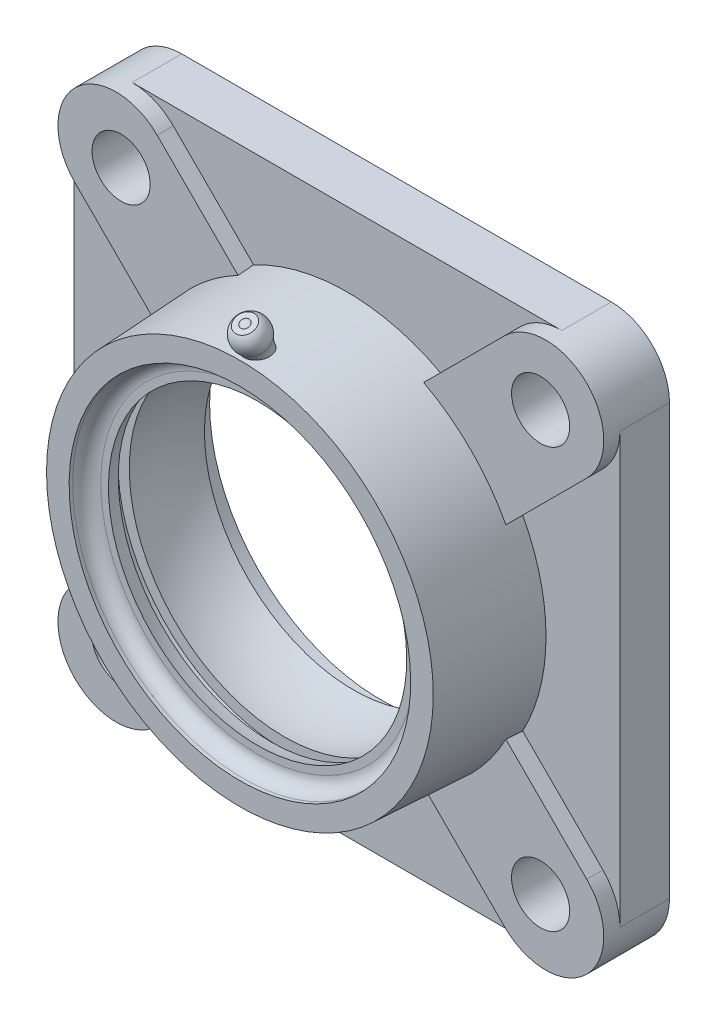
from build123d import *

# Parameters (mm, degrees)
SKETCH_1_R          = 5.75
EXTRUDE_686_DEPTH   = 9.8
SKETCH_2_R          = 5.75
EXTRUDE_1_DEPTH     = 13
CUT_EXTRUDE_3_DEPTH = 3.2
SKETCH_4_R          = 39.37
EXTRUDE_2_DEPTH     = 21.2
EXTRUDE_2_TAPER     = 3


with BuildPart() as part:
    # 草图1 → Extrude 686 (new body)
    with BuildSketch(Plane.XY):
        with BuildLine():
            Line((-42.5, -54), (42.5, -54))
            ThreePointArc((42.5, -54), (50.631727984, -50.631727984), (54, -42.5))
            Line((54, -42.5), (54, 42.5))
            ThreePointArc((54, 42.5), (50.631727984, 50.631727984), (42.5, 54))
            Line((42.5, 54), (-42.5, 54))
            ThreePointArc((-42.5, 54), (-50.631727984, 50.631727984), (-54, 42.5))
            Line((-54, 42.5), (-54, -42.5))
            ThreePointArc((-54, -42.5), (-50.631727984, -50.631727984), (-42.5, -54))
        make_face()
        with Locations((-41.5, -41.5)):
            Circle(SKETCH_1_R, mode=Mode.SUBTRACT)
        with Locations(Location((-41.5, 41.5, 0), (0, 0, 180))):
            Circle(SKETCH_1_R, mode=Mode.SUBTRACT)
        with Locations(Location((41.5, -41.5, 0), (0, 0, 180))):
            Circle(SKETCH_1_R, mode=Mode.SUBTRACT)
        with Locations((41.5, 41.5)):
            Circle(SKETCH_1_R, mode=Mode.SUBTRACT)
    extrude(amount=EXTRUDE_686_DEPTH)

    # 草图2 → 凸台-拉伸1 (add)
    # profile 1 of 4: a face of its own
    with BuildSketch(Plane.XY):
        with BuildLine():
            Line((-50.631727984, -34.368272016), (-18.763455967, -2.5))
            Line((-18.763455967, -2.5), (-2.5, -18.763455967))
            Line((-2.5, -18.763455967), (-34.368272016, -50.631727984))
            ThreePointArc((-34.368272016, -50.631727984), (-50.631727984, -50.631727984), (-50.631727984, -34.368272016))
        make_face()
        with Locations((-41.5, -41.5)):
            Circle(SKETCH_2_R, mode=Mode.SUBTRACT)
    # profile 2 of 4: a face of its own
    with BuildSketch(Plane.XY):
        with BuildLine():
            Line((-18.763455967, 2.5), (-2.5, 18.763455967))
            Line((-2.5, 18.763455967), (-34.368272016, 50.631727984))
            ThreePointArc((-34.368272016, 50.631727984), (-50.631727984, 50.631727984), (-50.631727984, 34.368272016))
            Line((-50.631727984, 34.368272016), (-18.763455967, 2.5))
        make_face()
        with Locations(Location((-41.5, 41.5, 0), (0, 0, 180))):
            Circle(SKETCH_2_R, mode=Mode.SUBTRACT)
    # profile 3 of 4: a face of its own
    with BuildSketch(Plane.XY):
        with BuildLine():
            Line((2.5, -18.763455967), (34.368272016, -50.631727984))
            ThreePointArc((34.368272016, -50.631727984), (50.631727984, -50.631727984), (50.631727984, -34.368272016))
            Line((50.631727984, -34.368272016), (18.763455967, -2.5))
            Line((18.763455967, -2.5), (2.5, -18.763455967))
        make_face()
        with Locations(Location((41.5, -41.5, 0), (0, 0, 180))):
            Circle(SKETCH_2_R, mode=Mode.SUBTRACT)
    # profile 4 of 4: a face of its own
    with BuildSketch(Plane.XY):
        with BuildLine():
            Line((2.5, 18.763455967), (34.368272016, 50.631727984))
            ThreePointArc((34.368272016, 50.631727984), (50.631727984, 50.631727984), (50.631727984, 34.368272016))
            Line((50.631727984, 34.368272016), (18.763455967, 2.5))
            Line((18.763455967, 2.5), (2.5, 18.763455967))
        make_face()
        with Locations((41.5, 41.5)):
            Circle(SKETCH_2_R, mode=Mode.SUBTRACT)
    extrude(amount=EXTRUDE_1_DEPTH)

    # 草图3 → 切除-拉伸3 (cut)
    with BuildSketch(Plane.XY):
        with BuildLine():
            Line((-26.757388349, 48.125), (26.757388349, 48.125))
            ThreePointArc((26.757388349, 48.125), (29.193644663, 46.875615655), (29.600687311, 44.168103448))
            ThreePointArc((29.600687311, 44.168103448), (30.719443759, 34.450973663), (38.913793103, 29.10991889))
            ThreePointArc((38.913793103, 29.10991889), (40.762894088, 28.108189877), (41.5, 26.138593384))
            Line((41.5, 26.138593384), (41.5, 12.625))
            ThreePointArc((41.5, 12.625), (42.378679656, 10.503679656), (44.5, 9.625))
            Line((44.5, 9.625), (45.125, 9.625))
            ThreePointArc((45.125, 9.625), (47.246320344, 8.746320344), (48.125, 6.625))
            Line((48.125, 6.625), (48.125, -26.757388349))
            ThreePointArc((48.125, -26.757388349), (46.875615655, -29.193644663), (44.168103448, -29.600687311))
            ThreePointArc((44.168103448, -29.600687311), (32.368272016, -32.368272016), (29.600687311, -44.168103448))
            ThreePointArc((29.600687311, -44.168103448), (29.193644663, -46.875615655), (26.757388349, -48.125))
            Line((26.757388349, -48.125), (-26.757388349, -48.125))
            ThreePointArc((-26.757388349, -48.125), (-29.193644663, -46.875615655), (-29.600687311, -44.168103448))
            ThreePointArc((-29.600687311, -44.168103448), (-30.719443759, -34.450973663), (-38.913793103, -29.10991889))
            ThreePointArc((-38.913793103, -29.10991889), (-40.762894088, -28.108189877), (-41.5, -26.138593384))
            Line((-41.5, -26.138593384), (-41.5, -12.625))
            ThreePointArc((-41.5, -12.625), (-42.378679656, -10.503679656), (-44.5, -9.625))
            Line((-44.5, -9.625), (-45.125, -9.625))
            ThreePointArc((-45.125, -9.625), (-47.246320344, -8.746320344), (-48.125, -6.625))
            Line((-48.125, -6.625), (-48.125, 26.757388349))
            ThreePointArc((-48.125, 26.757388349), (-46.875615655, 29.193644663), (-44.168103448, 29.600687311))
            ThreePointArc((-44.168103448, 29.600687311), (-32.368272016, 32.368272016), (-29.600687311, 44.168103448))
            ThreePointArc((-29.600687311, 44.168103448), (-29.193644663, 46.875615655), (-26.757388349, 48.125))
        make_face()
    extrude(amount=CUT_EXTRUDE_3_DEPTH, mode=Mode.SUBTRACT)

    # 草图4 → 凸台-拉伸2 (add)
    with BuildSketch(Plane.XY.offset(9.8)):
        Circle(SKETCH_4_R)
    extrude(amount=EXTRUDE_2_DEPTH, taper=EXTRUDE_2_TAPER)

    # 草图5 → 切除-旋转1 (revolve, cut)
    with BuildSketch(Plane(origin=(0, 0, 0), x_dir=(0, 0, -1), z_dir=(1, 0, 0))):
        with BuildLine():
            Line((-31, 33.79), (-30.29, 33.79))
            ThreePointArc((-30.29, 33.79), (-28.31717208, 32.97282792), (-27.5, 31))
            Line((-27.5, 31), (-27.5, 29.508473359))
            ThreePointArc((-27.5, 29.508473359), (-26.174797201, 29.902720457), (-24.833333333, 30.237485933))
            Line((-24.833333333, 30.237485933), (-24.833333333, 32.97282792))
            Line((-24.833333333, 32.97282792), (-22.166666667, 32.97282792))
            Line((-22.166666667, 32.97282792), (-22.166666667, 30.718705847))
            ThreePointArc((-22.166666667, 30.718705847), (-15.265539033, 30.879163253), (-8.5, 29.508473359))
            Line((-8.5, 29.508473359), (-8.5, 31))
            ThreePointArc((-8.5, 31), (-7.68282792, 32.97282792), (-5.71, 33.79))
            Line((-5.71, 33.79), (0, 33.79))
            Line((0, 33.79), (0, 0))
            Line((0, 0), (-31, 0))
            Line((-31, 0), (-31, 33.79))
        make_face()
    revolve(axis=Axis((0, 0, 0), (0, 0, 1)), mode=Mode.SUBTRACT)

    # 草图6 → 凸台-旋转1 (revolve)
    with BuildSketch(Plane(origin=(0, 0, 0), x_dir=(0, 0, -1), z_dir=(1, 0, 0))):
        with BuildLine():
            Line((-28.142278533, 34.39), (-25.967139844, 35.404283828))
            Line((-25.967139844, 35.404283828), (-30.121450593, 44.313231979))
            ThreePointArc((-30.121450593, 44.313231979), (-30.524648689, 44.039654202), (-30.821450593, 43.653231979))
            Line((-30.821450593, 43.653231979), (-31.806295837, 43.193991099))
            ThreePointArc((-31.806295837, 43.193991099), (-32.109703255, 41.142115004), (-31.110252397, 39.324603091))
            ThreePointArc((-31.110252397, 39.324603091), (-30.068637739, 38.160089016), (-29.27322829, 36.815329582))
            Line((-29.27322829, 36.815329582), (-28.142278533, 34.39))
        make_face()
    revolve(axis=Axis((0, 32.97282792, 24.833333333), (0, 0.9063077870366524, 0.42261826174069445)))


solid = part.part
